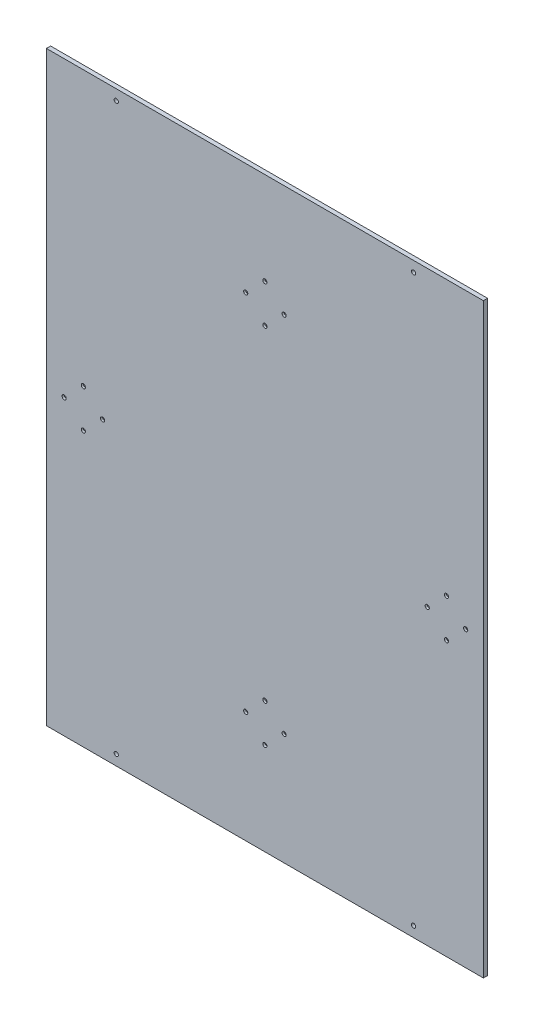
from build123d import *

# Parameters (mm, degrees)
SKETCH2_W           = 625.68542495
SKETCH2_H           = 840
BOSS_EXTRUDE1_DEPTH = 6
SKETCH3_R           = 3
CUT_EXTRUDE1_DEPTH  = 3
CUT_EXTRUDE2_DEPTH  = 36


with BuildPart() as part:
    # Sketch2 → Boss-Extrude1 (new body)
    with BuildSketch(Plane.XY):
        with Locations((438.821917673, -373.378193942)):
            Rectangle(SKETCH2_W, SKETCH2_H)
    extrude(amount=BOSS_EXTRUDE1_DEPTH)

    # Sketch3 → Cut-Extrude1 (cut)
    with BuildSketch(Plane.XY.offset(6)):
        with Locations((438.821917673, -660.878193942)):
            Circle(SKETCH3_R)
        with Locations((411.321917673, -633.378193942)):
            Circle(SKETCH3_R)
        with Locations((438.821917673, -605.878193942)):
            Circle(SKETCH3_R)
        with Locations((466.321917673, -633.378193942)):
            Circle(SKETCH3_R)
        with Locations((151.321917673, -373.378193942)):
            Circle(SKETCH3_R)
        with Locations((178.821917673, -345.878193942)):
            Circle(SKETCH3_R)
        with Locations((206.321917673, -373.378193942)):
            Circle(SKETCH3_R)
        with Locations((178.821917673, -400.878193942)):
            Circle(SKETCH3_R)
        with Locations((438.821917673, -140.878193942)):
            Circle(SKETCH3_R)
        with Locations((411.321917673, -113.378193942)):
            Circle(SKETCH3_R)
        with Locations((438.821917673, -85.878193942)):
            Circle(SKETCH3_R)
        with Locations((466.321917673, -113.378193942)):
            Circle(SKETCH3_R)
        with Locations((698.821917673, -400.878193942)):
            Circle(SKETCH3_R)
        with Locations((671.321917673, -373.378193942)):
            Circle(SKETCH3_R)
        with Locations((698.821917673, -345.878193942)):
            Circle(SKETCH3_R)
        with Locations((726.321917673, -373.378193942)):
            Circle(SKETCH3_R)
    extrude(amount=-CUT_EXTRUDE1_DEPTH, mode=Mode.SUBTRACT)

    # Sketch6 → Cut-Extrude2 (cut)
    with BuildSketch(Plane.XY.offset(6)):
        with BuildLine():
            ThreePointArc((654.664630148, -778.378193942), (651.664630148, -775.378193942), (648.664630148, -778.378193942))
            Line((648.664630148, -778.378193942), (654.664630148, -778.378193942))
        make_face()
        with BuildLine():
            Line((654.664630148, -778.378193942), (648.664630148, -778.378193942))
            ThreePointArc((648.664630148, -778.378193942), (651.664630148, -781.378193942), (654.664630148, -778.378193942))
        make_face()
        with BuildLine():
            ThreePointArc((228.979205198, -778.378193942), (225.979205198, -775.378193942), (222.979205198, -778.378193942))
            Line((222.979205198, -778.378193942), (228.979205198, -778.378193942))
        make_face()
        with BuildLine():
            Line((228.979205198, -778.378193942), (222.979205198, -778.378193942))
            ThreePointArc((222.979205198, -778.378193942), (225.979205198, -781.378193942), (228.979205198, -778.378193942))
        make_face()
        with BuildLine():
            ThreePointArc((222.979205198, 31.621806058), (225.979205198, 28.621806058), (228.979205198, 31.621806058))
            Line((228.979205198, 31.621806058), (222.979205198, 31.621806058))
        make_face()
        with BuildLine():
            Line((222.979205198, 31.621806058), (228.979205198, 31.621806058))
            ThreePointArc((228.979205198, 31.621806058), (225.979205198, 34.621806058), (222.979205198, 31.621806058))
        make_face()
        with BuildLine():
            Line((648.664630148, 31.621806058), (651.664630148, 31.621806058))
            Line((651.664630148, 31.621806058), (654.664630148, 31.621806058))
            ThreePointArc((654.664630148, 31.621806058), (651.664630148, 34.621806058), (648.664630148, 31.621806058))
        make_face()
        with BuildLine():
            Line((654.664630148, 31.621806058), (651.664630148, 31.621806058))
            Line((651.664630148, 31.621806058), (648.664630148, 31.621806058))
            ThreePointArc((648.664630148, 31.621806058), (651.664630148, 28.621806058), (654.664630148, 31.621806058))
        make_face()
    extrude(amount=-CUT_EXTRUDE2_DEPTH, mode=Mode.SUBTRACT)


solid = part.part
